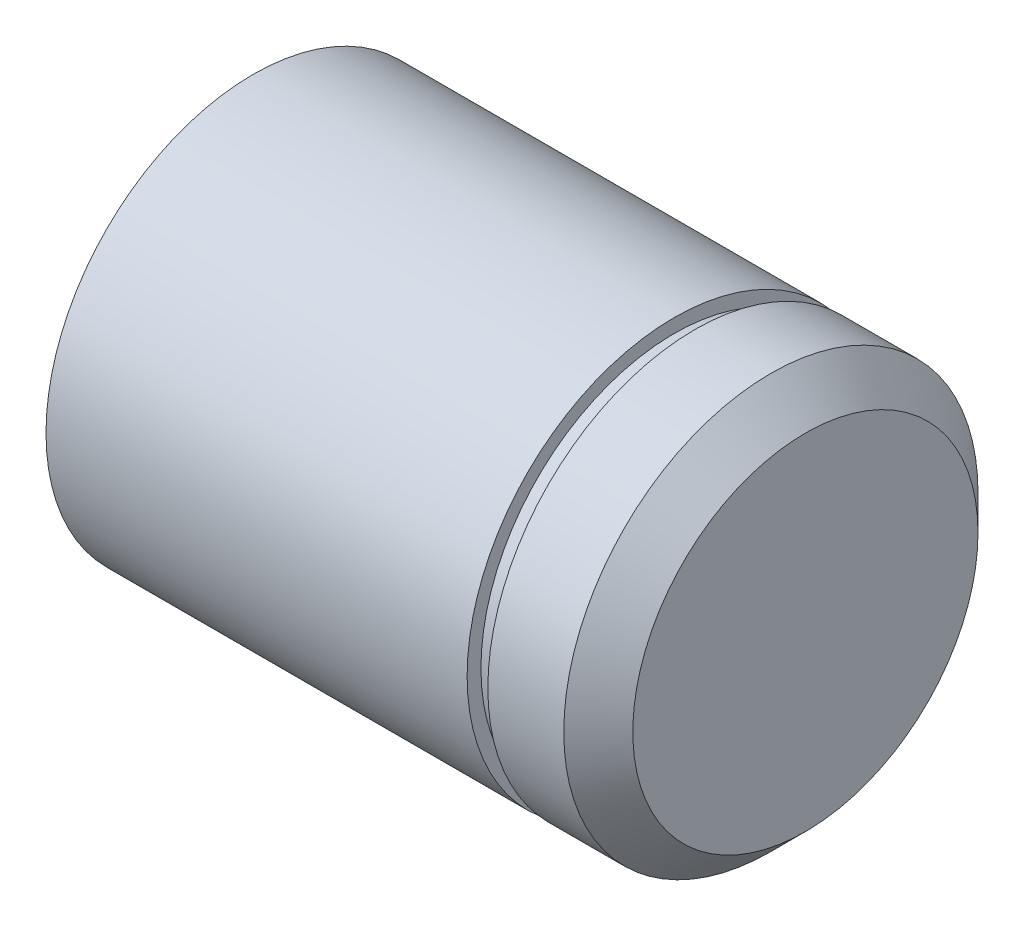
from build123d import *

# Parameters (mm, degrees)
SKETCH1_R             = 3
BOSS_EXTRUDE1_DEPTH   = 8
CHAMFER1_SIZE         = 0.5
M3_TAPPED_HOLE1_D     = 2.5
M3_TAPPED_HOLE1_DEPTH = 6.5
M3_TAPPED_HOLE1_TIP   = 0.751075774
SKETCH3_W             = 0.3
SKETCH3_H             = 0.2


with BuildPart() as part:
    # Sketch1 → Boss-Extrude1 (new body)
    with BuildSketch(Plane(origin=(0, 0, 0), x_dir=(0, 0, -1), z_dir=(1, 0, 0))):
        Circle(SKETCH1_R)
    extrude(amount=BOSS_EXTRUDE1_DEPTH)

    # Chamfer1
    chamfer1_edges = [part.edges().sort_by_distance(p)[0] for p in [
        (8, 0, 3),
    ]]
    chamfer(chamfer1_edges, length=CHAMFER1_SIZE)

    # M3 Tapped Hole1
    with Locations(Plane(origin=(0, 0, 0), x_dir=(0, 0, -1), z_dir=(-1, 0, 0))):
        with Locations((0, 0)):
            Hole(M3_TAPPED_HOLE1_D / 2, depth=M3_TAPPED_HOLE1_DEPTH)
            with Locations((0, 0, -(M3_TAPPED_HOLE1_DEPTH + M3_TAPPED_HOLE1_TIP / 2))):  # 118° drill point
                Cone(0, M3_TAPPED_HOLE1_D / 2, M3_TAPPED_HOLE1_TIP, mode=Mode.SUBTRACT)

    # Sketch3 → Cut-Revolve1 (revolve, cut)
    with BuildSketch(Plane(origin=(0, 0, 0), x_dir=(1, 0, 0), z_dir=(0, 1, 0)), mode=Mode.PRIVATE) as cut_revolve1_sk:
        with Locations((6.25, 2.9)):
            Rectangle(SKETCH3_W, SKETCH3_H)
    revolve(cut_revolve1_sk.sketch.rotate(Axis((0, 0, 0), (1, 0, 0)), 180), axis=Axis((0, 0, 0), (1, 0, 0)), mode=Mode.SUBTRACT)


solid = part.part
